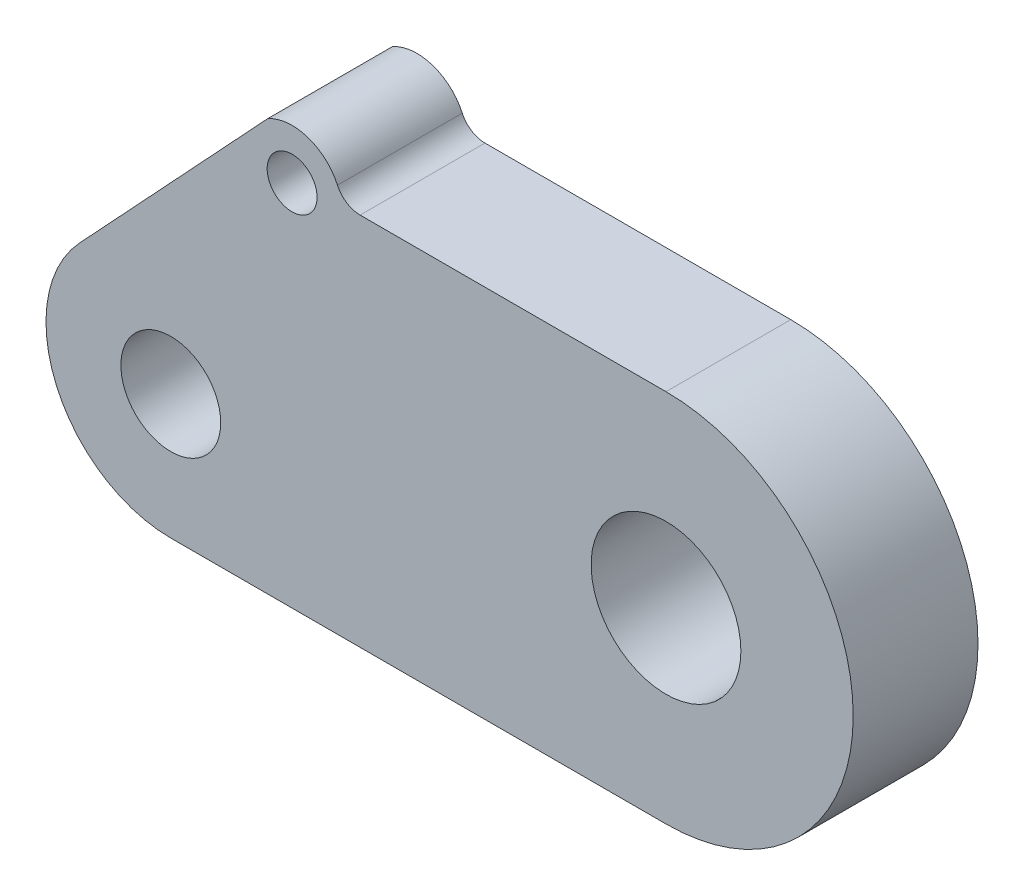
SolidWorks part; units mm, degrees
ref_plane "Front Plane" through (0, 0, 0) normal (0, 0, 1) x (1, 0, 0)
ref_plane "Top Plane" through (0, 0, 0) normal (0, 1, 0) x (1, 0, 0)
ref_plane "Right Plane" through (0, 0, 0) normal (1, 0, 0) x (0, 0, -1)
other "Configuration Table"
sketch "Sketch1" plane through (0, 0, 0) normal (0, 0, 1) x (1, 0, 0)
  line L0 (-19.84, -7.5) -> (0, -7.5)
  line L1 (0, 7.5) -> (-12.2528, 7.5)
  line L2 (-15.9575, 8.9948) -> (-23.4968, 0.91)
  circle A0 centre (0, 0) radius 3
  arc A1 (0, -7.5) -> (0, 7.5) centre (0, 0) ccw
  circle A2 centre (-14.98, 7.25) radius 1
  circle A3 centre (-19.84, -2.5) radius 2
  arc A4 (-13.1619, 8.0833) -> (-15.9575, 8.9948) centre (-14.98, 7.25) ccw
  arc A5 (-23.4968, 0.91) -> (-19.84, -7.5) centre (-19.84, -2.5) ccw
  arc A6 (-13.1619, 8.0833) -> (-12.2528, 7.5) centre (-12.2528, 8.5) ccw
  dimension "D1" = 6
  dimension "D4" = 4
  dimension "D8" = 2
  dimension "D9" = 4
  dimension "D11" = 10
  dimension "D12" = 1
  dimension "D2" = 7.5
  dimension "D3" = 5
  dimension "D5" = 19.84
  dimension "D6" = 14.75
  dimension "D7" = 14.98
  dimension "D10" = 47
extrude "Boss-Extrude1" add sketch "Sketch1" along normal blind 5
